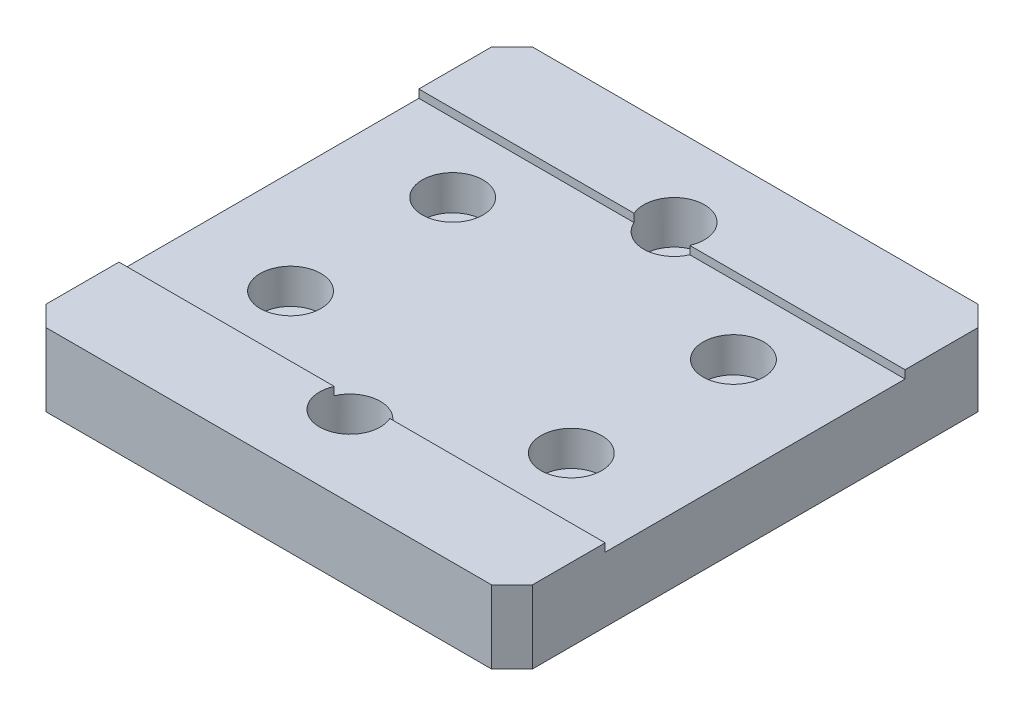
from build123d import *

# Parameters (mm, degrees)
SKETCH_1_W                   = 120
SKETCH_1_H                   = 120
EXTRUDE_1_DEPTH              = 18
HOLE_WIZARD_M8_3_D           = 9
HOLE_WIZARD_M8_3_CBORE_D     = 15
HOLE_WIZARD_M8_3_CBORE_DEPTH = 10.6
SKETCH_11_W                  = 120
SKETCH_11_H                  = 74
CUT_EXTRUDE_2_DEPTH          = 2
CHAMFER_1_SIZE               = 5


with BuildPart() as part:
    # 草图1 → 凸台-拉伸1 (new body)
    with BuildSketch(Plane(origin=(0, 0, 0), x_dir=(1, 0, 0), z_dir=(0, 1, 0))):
        Rectangle(SKETCH_1_W, SKETCH_1_H)
    extrude(amount=EXTRUDE_1_DEPTH)

    # M8 六角凹头螺钉的柱形沉头孔3 (through all)
    with Locations(Plane(origin=(0, 18, 0), x_dir=(1, 0, 0), z_dir=(0, 1, 0))):
        with Locations((0, 40), (-34.641016151, 20), (-34.641016151, -20), (0, -40), (34.641016151, -20), (34.641016151, 20)):
            CounterBoreHole(HOLE_WIZARD_M8_3_D / 2, HOLE_WIZARD_M8_3_CBORE_D / 2, HOLE_WIZARD_M8_3_CBORE_DEPTH)

    # 草图11 → 切除-拉伸2 (cut)
    with BuildSketch(Plane(origin=(0, 18, 0), x_dir=(1, 0, 0), z_dir=(0, 1, 0))):
        Rectangle(SKETCH_11_W, SKETCH_11_H)
    extrude(amount=-CUT_EXTRUDE_2_DEPTH, mode=Mode.SUBTRACT)

    # 倒角1
    chamfer_1_edges = [part.edges().sort_by_distance(p)[0] for p in [
        (60, 9, 60),
        (-60, 9, 60),
        (-60, 9, -60),
        (60, 9, -60),
    ]]
    chamfer(chamfer_1_edges, length=CHAMFER_1_SIZE)


solid = part.part
